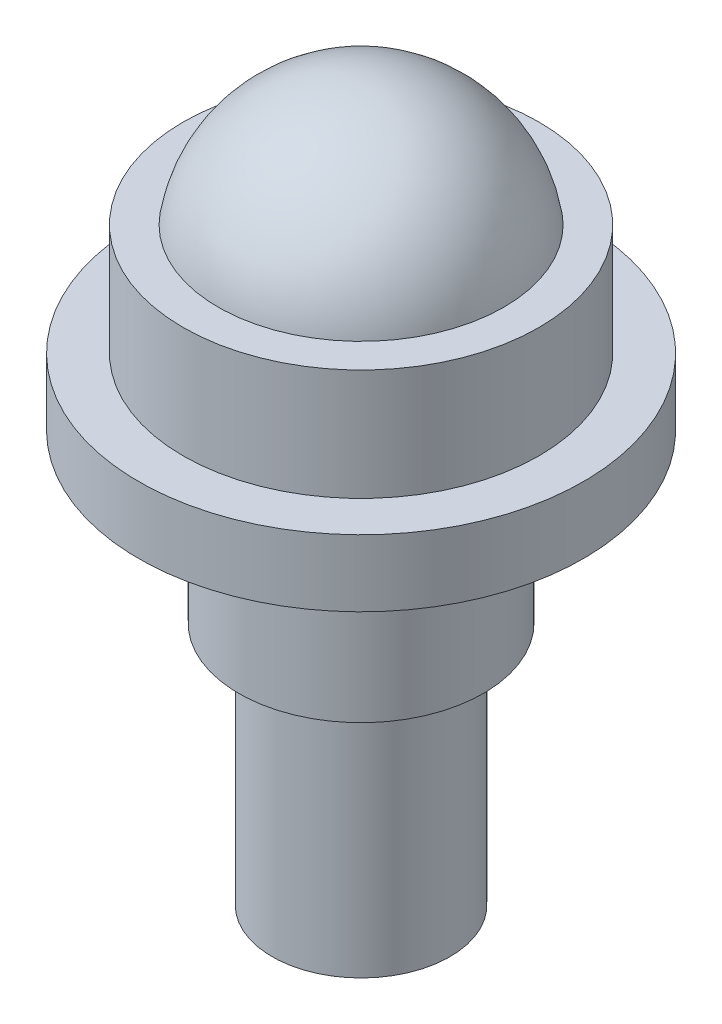
from build123d import *

# Parameters (mm, degrees)
SKETCH2_R           = 11
BOSS_EXTRUDE1_DEPTH = 15
SKETCH3_R           = 8
BOSS_EXTRUDE2_DEPTH = 22


with BuildPart() as part:
    # Sketch1 → Revolve1 (revolve)
    with BuildSketch(Plane.XY, mode=Mode.PRIVATE) as revolve1_sk:
        with BuildLine():
            Line((-12.845232579, 16), (-16, 16))
            Line((-16, 16), (-16, 6))
            Line((-16, 6), (-20, 6))
            Line((-20, 6), (-20, 0))
            Line((-20, 0), (0, 0))
            Line((0, 0), (0, 27))
            ThreePointArc((0, 27), (-8.455767263, 23.874208829), (-12.845232579, 16))
        make_face()
    revolve(revolve1_sk.sketch.rotate(Axis((0, 0, 0), (0, 1, 0)), 270), axis=Axis((0, 0, 0), (0, 1, 0)))

    # Sketch2 → Boss-Extrude1 (add)
    with BuildSketch(Plane(origin=(0, 0, 0), x_dir=(-1, 0, 0), z_dir=(0, -1, 0))):
        with Locations(Location((0, 0, 0), (0, 0, 90))):
            Circle(SKETCH2_R)
    extrude(amount=BOSS_EXTRUDE1_DEPTH)

    # Sketch3 → Boss-Extrude2 (add)
    with BuildSketch(Plane(origin=(0, -15, 0), x_dir=(-1, 0, 0), z_dir=(0, -1, 0))):
        with Locations(Location((0, 0, 0), (0, 0, 90))):
            Circle(SKETCH3_R)
    extrude(amount=BOSS_EXTRUDE2_DEPTH)


solid = part.part
